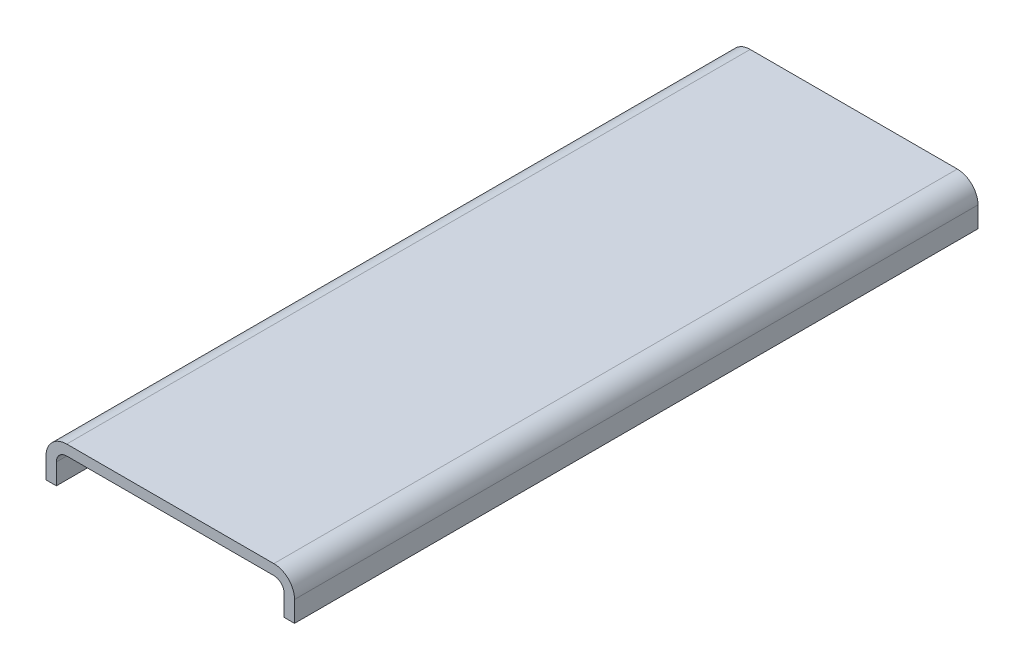
SolidWorks part; units mm, degrees
ref_plane "前视基准面" through (0, 0, 0) normal (0, 0, 1) x (1, 0, 0)
ref_plane "上视基准面" through (0, 0, 0) normal (0, 1, 0) x (1, 0, 0)
ref_plane "右视基准面" through (0, 0, 0) normal (1, 0, 0) x (0, 0, -1)
sketch "草图1" plane through (0, 0, 0) normal (0, 0, 1) x (1, 0, 0)
  line L0 (10, 0) -> (110, 0)
  line L1 (120, -10) -> (120, -20)
  line L2 (0, -10) -> (0, -20)
  line L3 (5, -10) -> (5, -20)
  line L4 (10, -5) -> (110, -5)
  line L5 (115, -10) -> (115, -20)
  line L6 (0, -20) -> (5, -20)
  line L7 (115, -20) -> (120, -20)
  arc A0 (120, -10) -> (110, 0) centre (110, -10) ccw
  arc A1 (10, 0) -> (0, -10) centre (10, -10) ccw
  arc A2 (10, -5) -> (5, -10) centre (10, -10) ccw
  arc A3 (115, -10) -> (110, -5) centre (110, -10) ccw
  point P9 (0, 0)
  dimension "D1" = 10
  dimension "D2" = 5
extrude "凸台-拉伸1" add sketch "草图1" along normal blind 320
sketch "草图2" plane through (0, 0, 0) normal (0, 0, -1) x (-1, 0, 0)
  line L16 (-120, -20) -> (-115, -20)
  line L17 (-115, -20) -> (-115, -10)
  line L18 (-110, -5) -> (-10, -5)
  line L19 (-5, -10) -> (-5, -20)
  line L20 (-5, -20) -> (0, -20)
  line L21 (0, -20) -> (0, -10)
  line L22 (-10, 0) -> (-110, 0)
  line L23 (-120, -10) -> (-120, -20)
  line L24 (-120, -20) -> (-115, -20)
  line L25 (-115, -20) -> (-115, -10)
  line L26 (-110, -5) -> (-10, -5)
  line L27 (-5, -10) -> (-5, -20)
  line L28 (-5, -20) -> (0, -20)
  line L29 (0, -20) -> (0, -10)
  line L30 (-10, 0) -> (-110, 0)
  line L31 (-120, -10) -> (-120, -20)
  arc A8 (-110, -5) -> (-115, -10) centre (-110, -10) ccw
  arc A9 (-5, -10) -> (-10, -5) centre (-10, -10) ccw
  arc A10 (0, -10) -> (-10, 0) centre (-10, -10) ccw
  arc A11 (-110, 0) -> (-120, -10) centre (-110, -10) ccw
  arc A12 (-110, -5) -> (-115, -10) centre (-110, -10) ccw
  arc A13 (-5, -10) -> (-10, -5) centre (-10, -10) ccw
  arc A14 (0, -10) -> (-10, 0) centre (-10, -10) ccw
  arc A15 (-110, 0) -> (-120, -10) centre (-110, -10) ccw
  dimension "D1" = 0
extrude "凸台-拉伸2" add sketch "草图2" along normal blind 10
